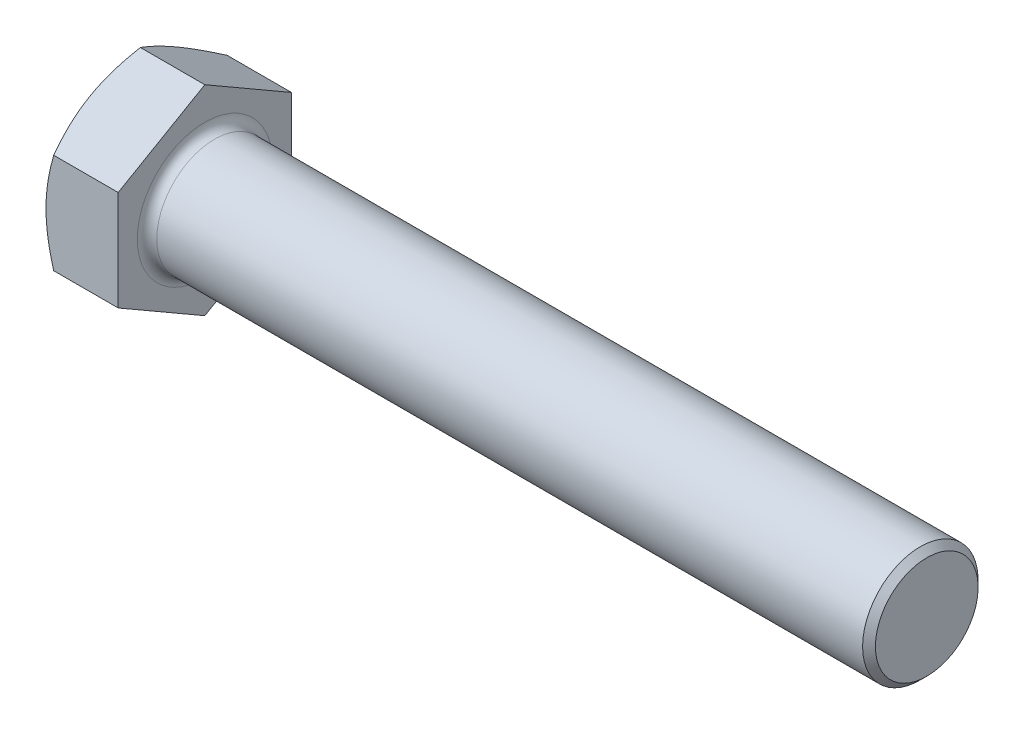
SolidWorks part; units mm, degrees
material "Q235"
ref_plane "Front Plane" through (0, 0, 0) normal (0, 0, 1) x (1, 0, 0)
ref_plane "Top Plane" through (0, 0, 0) normal (0, 1, 0) x (1, 0, 0)
ref_plane "Right Plane" through (0, 0, 0) normal (1, 0, 0) x (0, 0, -1)
sketch "Sketch1" plane through (0, 0, 0) normal (0, 0, 1) x (1, 0, 0)
  line L0 (0, 0) -> (110, 0) construction
  line L1 (0, 0) -> (0, 13.085)
  line L2 (0, 13.085) -> (10, 13.085)
  line L3 (10, 13.085) -> (10, 0)
  line L4 (10, 8) -> (110, 8)
  line L5 (110, 8) -> (110, 0)
  line L6 (0, 12) -> (0.6264, 13.085)
  line L7 (106, 8) -> (106, 0)
  line L8 (16, 8) -> (16, 0)
  line L9 (10, 7.3505) -> (110, 7.3505)
  line L10 (110, 6.9175) -> (10, 6.9175)
  line L11 (9.2, 11.7) -> (10, 10.9)
  line L12 (9.2, 13.085) -> (9.2, 0)
  line L13 (9.9, 11) -> (9.9, 0) construction
  arc A0 (10, 9.35) -> (11.35, 8) centre (11.35, 9.35) ccw
  point P12 (108, 0)
  point P13 (3.52, 13.085)
  point P14 (10, 9.35)
  point P24 (10, 11)
  dimension "D1" = 0.1
  dimension "r" = 1.35
  dimension "k" = 10
  dimension "D2" = 45
  dimension "β" = 30
  dimension "e" = 26.17
  dimension "s" = 24
  dimension "d" = 16
  dimension "l" = 100
  dimension "D52" = 4
  dimension "P" = 2
  dimension "kw" = 6.48
  dimension "da" = 18.7
  dimension "a" = 6
  dimension "ds" = 14.701
  dimension "D61" = 13.835
  dimension "dw" = 22
  dimension "c" = 0.8
sketch "Sketch2" plane through (0, 0, 0) normal (1, 0, 0) x (0, 0, -1)
  line L1 (0, 13.8564) -> (-12, 6.9282)
  line L2 (-12, 6.9282) -> (-12, -6.9282)
  line L3 (-12, -6.9282) -> (0, -13.8564)
  line L4 (0, -13.8564) -> (12, -6.9282)
  line L5 (12, -6.9282) -> (12, 6.9282)
  line L6 (12, 6.9282) -> (0, 13.8564)
  circle A0 centre (0, 0) radius 12 construction
sketch "Sketch3" plane through (0, 0, 0) normal (1, 0, 0) x (0, 0, -1)
  line L0 (12, 6.9282) -> (0, 13.8564) construction
  line L1 (0, 13.8564) -> (-12, 6.9282) construction
  line L2 (-12, 6.9282) -> (-12, -6.9282) construction
  line L3 (12, -6.9282) -> (12, 6.9282) construction
  line L4 (0, -13.8564) -> (12, -6.9282) construction
  line L5 (-12, -6.9282) -> (0, -13.8564) construction
  line L6 (12, 6.9282) -> (0, 13.8564)
  line L7 (0, 13.8564) -> (-12, 6.9282)
  line L8 (-12, 6.9282) -> (-12, -6.9282)
  line L9 (12, -6.9282) -> (12, 6.9282)
  line L10 (0, -13.8564) -> (12, -6.9282)
  line L11 (-12, -6.9282) -> (0, -13.8564)
extrude "Boss-Extrude1" add sketch "Sketch3" along normal up to vertex (10 mm away) up to point (10, 13.085, 0)
sketch "Sketch4" plane through (0, 0, 0) normal (-1, 0, 0) x (0, 0, 1)
  circle A0 centre (0, 0) radius 12 construction
  circle A1 centre (0, 0) radius 12
  circle A2 centre (0, 0) radius 26.17
  dimension "D1" = 52.34
extrude "Cut-Extrude1" cut sketch "Sketch4" against normal blind 1.25 draft 60
sketch "Sketch5" plane through (0, 0, 0) normal (0, 0, 1) x (1, 0, 0)
  line L0 (10, 8) -> (110, 8) construction
  line L1 (110, 8) -> (110, 0) construction
  line L2 (0, 0) -> (110, 0) construction
  line L3 (11.35, 8) -> (110, 8)
  line L4 (110, 8) -> (110, 0)
  line L5 (10, 0) -> (110, 0)
  line L6 (10, 9.35) -> (10, 0)
  arc A0 (10, 9.35) -> (11.35, 8) centre (11.35, 9.35) ccw construction
  arc A1 (10, 9.35) -> (11.35, 8) centre (11.35, 9.35) ccw
revolve "Revolve1" add sketch "Sketch5" angle 360 about L5
cosmetic thread "Cosmetic Thread2" parameters "D1"=49, "D2"=13.835
chamfer "Chamfer2" distance 0.8889 angle 45 1 edges at (110, 0, 8)
sketch "Sketch7" plane through (0, 0, 0) normal (0, 0, 1) x (1, 0, 0)
  line L0 (10, 10.9) -> (9.2, 11.7)
  line L1 (9.2, 11.7) -> (9.2, 26.17)
  line L2 (9.2, 26.17) -> (10, 26.17)
  line L3 (10, 26.17) -> (10, 10.9)
  line L4 (0, 0) -> (110, 0) construction
  line L5 (0, 0) -> (110, 0) construction
  dimension "D1" = 52.34
revolve "Cut-Revolve1" [suppressed] cut sketch "Sketch7" angle 360 mid plane about L5
sketch "Sketch6" [suppressed] plane through (0, 0, 0) normal (0, 0, 1) x (1, 0, 0)
  line L0 (5.9, 0) -> (5.9, 2.5) construction
  line L1 (5.9, 2.5) -> (13.5, 2.5)
  line L2 (13.5, 2.5) -> (13.5, 0)
  line L3 (5.9, 2.5) -> (4.069, 2.245)
  line L5 (3.5, 2.2402) -> (13.5, 2.2402) construction
  line L6 (3.5, 4.315) -> (3.5, 0) construction
  line L7 (3.5, 2.7402) -> (3.5, 0)
  line L8 (3.5, 0) -> (13.5, 0)
  arc A0 (4.069, 2.245) -> (3.5, 2.7402) centre (4, 2.7402) cw
  arc A1 (3.5, 3) -> (4, 2.5) centre (4, 3) ccw construction
revolve "Revolve2" add sketch "Sketch6" angle 360 about L8
cosmetic thread "Cosmetic Thread1" [suppressed] parameters "D1"=49, "D2"=13.835
chamfer "Chamfer1" [suppressed] distance 0.8889 angle 45
sketch "Sketch8" plane through (0, 0, 0) normal (0, 0, 1) x (1, 0, 0)
  line L0 (10, 10.9) -> (9.2, 11.7)
  line L1 (9.2, 11.7) -> (9.2, 26.17)
  line L2 (9.2, 26.17) -> (10, 26.17)
  line L3 (10, 26.17) -> (10, 10.9)
  line L4 (0, 0) -> (110, 0) construction
  line L5 (0, 0) -> (110, 0) construction
  dimension "D1" = 52.34
revolve "Cut-Revolve2" [suppressed] cut sketch "Sketch8" angle 360 mid plane about L5
